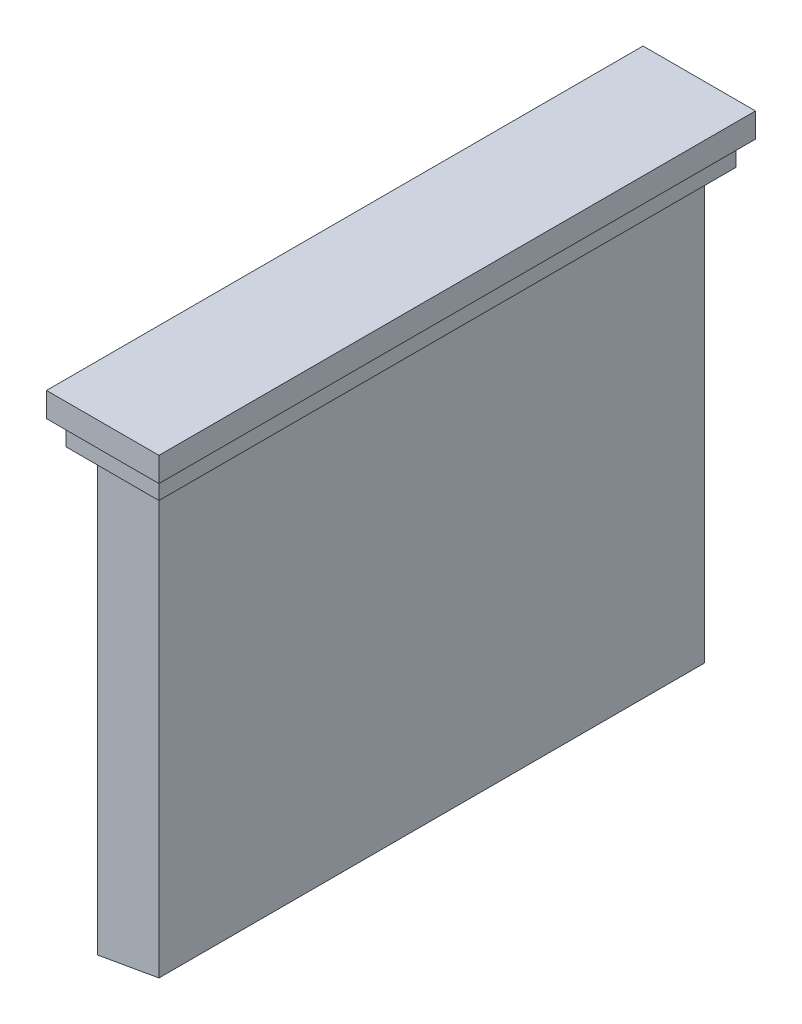
from build123d import *

# Parameters (mm, degrees)
SKETCH1_W           = 6.28
SKETCH1_H           = 55.78
BOSS_EXTRUDE1_DEPTH = 45
CUT_EXTRUDE1_DEPTH  = 72.737493684
SKETCH3_W           = 9.5
SKETCH3_H           = 59
BOSS_EXTRUDE2_DEPTH = 2.5
SKETCH4_W           = 11.5
SKETCH4_H           = 61
BOSS_EXTRUDE3_DEPTH = 2.5


with BuildPart() as part:
    # Sketch1 → Boss-Extrude1 (new body)
    with BuildSketch(Plane(origin=(0, 0, 0), x_dir=(1, 0, 0), z_dir=(0, 1, 0))):
        Rectangle(SKETCH1_W, SKETCH1_H)
    extrude(amount=BOSS_EXTRUDE1_DEPTH)

    # Sketch2 → Cut-Extrude1 (cut, through all)
    with BuildSketch(Plane.XY.offset(27.89)):
        Polygon((-3.14, 0), (3.14, 0), (3.14, 1.107333439), align=None)
    extrude(amount=-CUT_EXTRUDE1_DEPTH, mode=Mode.SUBTRACT)

    # Sketch3 → Boss-Extrude2 (add)
    with BuildSketch(Plane(origin=(0, 45, 0), x_dir=(1, 0, 0), z_dir=(0, 1, 0))):
        Rectangle(SKETCH3_W, SKETCH3_H)
    extrude(amount=BOSS_EXTRUDE2_DEPTH)

    # Sketch4 → Boss-Extrude3 (add)
    with BuildSketch(Plane(origin=(0, 47.5, 0), x_dir=(1, 0, 0), z_dir=(0, 1, 0))):
        Rectangle(SKETCH4_W, SKETCH4_H)
    extrude(amount=BOSS_EXTRUDE3_DEPTH)


solid = part.part
